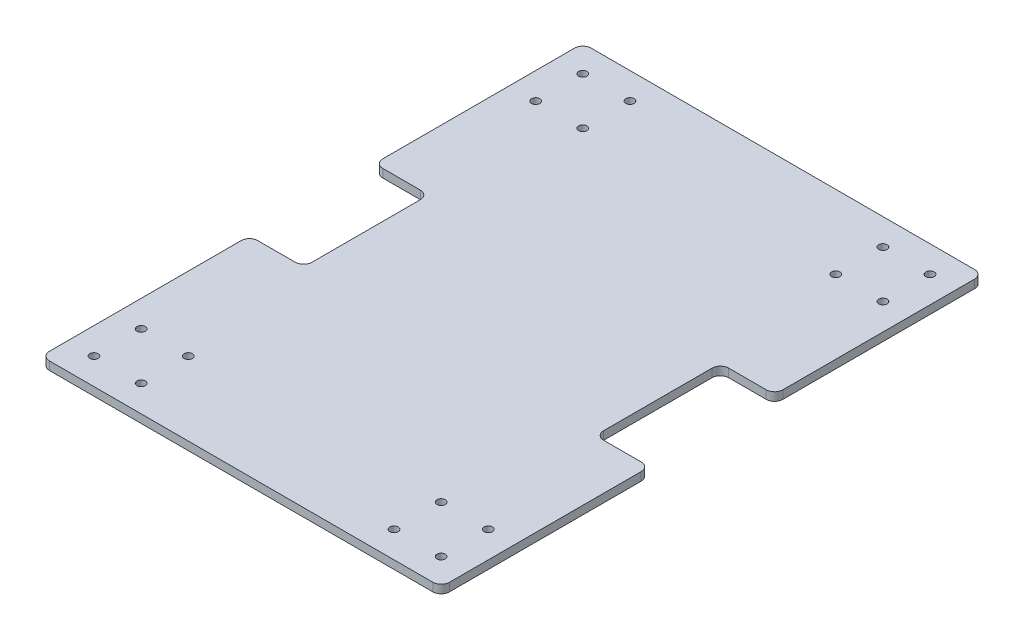
SolidWorks part; units mm, degrees
ref_plane "Front Plane" through (0, 0, 0) normal (0, 0, 1) x (1, 0, 0)
ref_plane "Top Plane" through (0, 0, 0) normal (0, 1, 0) x (1, 0, 0)
ref_plane "Right Plane" through (0, 0, 0) normal (1, 0, 0) x (0, 0, -1)
other "Configuration Table"
sketch "Sketch1" plane through (0, 0, 0) normal (0, 1, 0) x (1, 0, 0)
  line L1 (-240, 325) -> (240, 325)
  line L2 (-240, 325) -> (-240, -325)
  line L3 (-240, -325) -> (240, -325)
  line L4 (240, 325) -> (240, -325)
  line L5 (-240, 325) -> (240, -325) construction
  line L6 (-240, -325) -> (240, 325) construction
  point P0 (0, 0)
  dimension "D1" = 650
  dimension "D2" = 480
extrude "Boss-Extrude1" add sketch "Sketch1" along normal blind 10
sketch "Sketch3" plane through (0, 10, 0) normal (0, 1, 0) x (1, 0, 0)
  line L0 (0, 325) -> (0, -325) construction
  line L1 (240, 325) -> (-240, 325) construction
  line L2 (-240, -325) -> (240, -325) construction
  line L3 (-240, 0) -> (240, 0) construction
  line L4 (-240, 325) -> (-240, -325) construction
  line L5 (240, -325) -> (240, 325) construction
  line L6 (0, -325) -> (0, -225)
  line L26 (305, -75) -> (175, -75)
  line L27 (-305, 75) -> (-175, 75)
  line L28 (-305, 75) -> (-305, -75)
  line L29 (-305, -75) -> (-175, -75)
  line L30 (-175, 75) -> (-175, -75)
  line L31 (-305, 75) -> (-175, -75) construction
  line L32 (-305, -75) -> (-175, 75) construction
  line L33 (175, 75) -> (175, -75)
  line L34 (305, 75) -> (175, 75)
  line L35 (305, 75) -> (305, -75)
  dimension "D4" = 150
  dimension "D5" = 130
extrude "Cut-Extrude1" cut sketch "Sketch3" against normal blind 10
fillet "Fillet1" radius 10 8 edges at (-240, 5, -75) (-175, 5, -75) (-240, 5, 75) (-175, 5, 75) (240, 5, 75) (240, 5, -75) (175, 5, 75) (175, 5, -75)
sketch "Sketch5" plane through (0, 10, 0) normal (0, 1, 0) x (1, 0, 0)
  line L0 (0, 325) -> (0, -325) construction
  line L1 (240, 325) -> (-240, 325) construction
  line L2 (-240, -325) -> (240, -325) construction
  line L3 (-175, 0) -> (175, 0) construction
  line L4 (-175, 65) -> (-175, -65) construction
  line L5 (175, 65) -> (175, -65) construction
  line L6 (220, -305) -> (140, -305)
  line L7 (220, -225) -> (220, -305)
  line L8 (220, -225) -> (140, -225)
  line L9 (-220, -225) -> (-140, -225)
  line L10 (-220, -225) -> (-220, -305)
  line L11 (-220, -305) -> (-140, -305)
  line L12 (-140, -225) -> (-140, -305)
  line L13 (-220, -225) -> (-140, -305) construction
  line L14 (-220, -305) -> (-140, -225) construction
  line L15 (140, -225) -> (140, -305)
  line L16 (220, 305) -> (140, 305)
  line L17 (220, 225) -> (220, 305)
  line L18 (220, 225) -> (140, 225)
  line L19 (140, 225) -> (140, 305)
  line L20 (-140, 225) -> (-140, 305)
  line L21 (-220, 225) -> (-140, 225)
  line L22 (-220, 225) -> (-220, 305)
  line L23 (-220, 305) -> (-140, 305)
  line L24 (-180, -265) -> (-208.2843, -293.2843)
  circle A0 centre (-208.2843, -293.2843) radius 5
  circle A1 centre (-208.2843, -236.7157) radius 5
  circle A2 centre (-151.7157, -236.7157) radius 5
  circle A3 centre (-151.7157, -293.2843) radius 5
  circle A4 centre (208.2843, -293.2843) radius 5
  circle A5 centre (151.7157, -293.2843) radius 5
  circle A6 centre (151.7157, -236.7157) radius 5
  circle A7 centre (208.2843, -236.7157) radius 5
  circle A8 centre (-208.2843, 236.7157) radius 5
  circle A9 centre (208.2843, 293.2843) radius 5
  circle A10 centre (208.2843, 236.7157) radius 5
  circle A11 centre (151.7157, 293.2843) radius 5
  circle A12 centre (151.7157, 236.7157) radius 5
  circle A13 centre (-151.7157, 293.2843) radius 5
  circle A14 centre (-208.2843, 293.2843) radius 5
  circle A15 centre (-151.7157, 236.7157) radius 5
  point P40 (-180, -265)
  dimension "D6" = 10
  dimension "D1" = 140
  dimension "D2" = 20
  dimension "D3" = 80
  dimension "D4" = 80
  dimension "D5" = 40
  dimension "D7" = 4
fillet "Fillet3" radius 10 4 edges at (240, 5, -325) (-240, 5, -325) (240, 5, 325) (-240, 5, 325)
extrude "Cut-Extrude2" cut sketch "Sketch5" against normal blind 10
